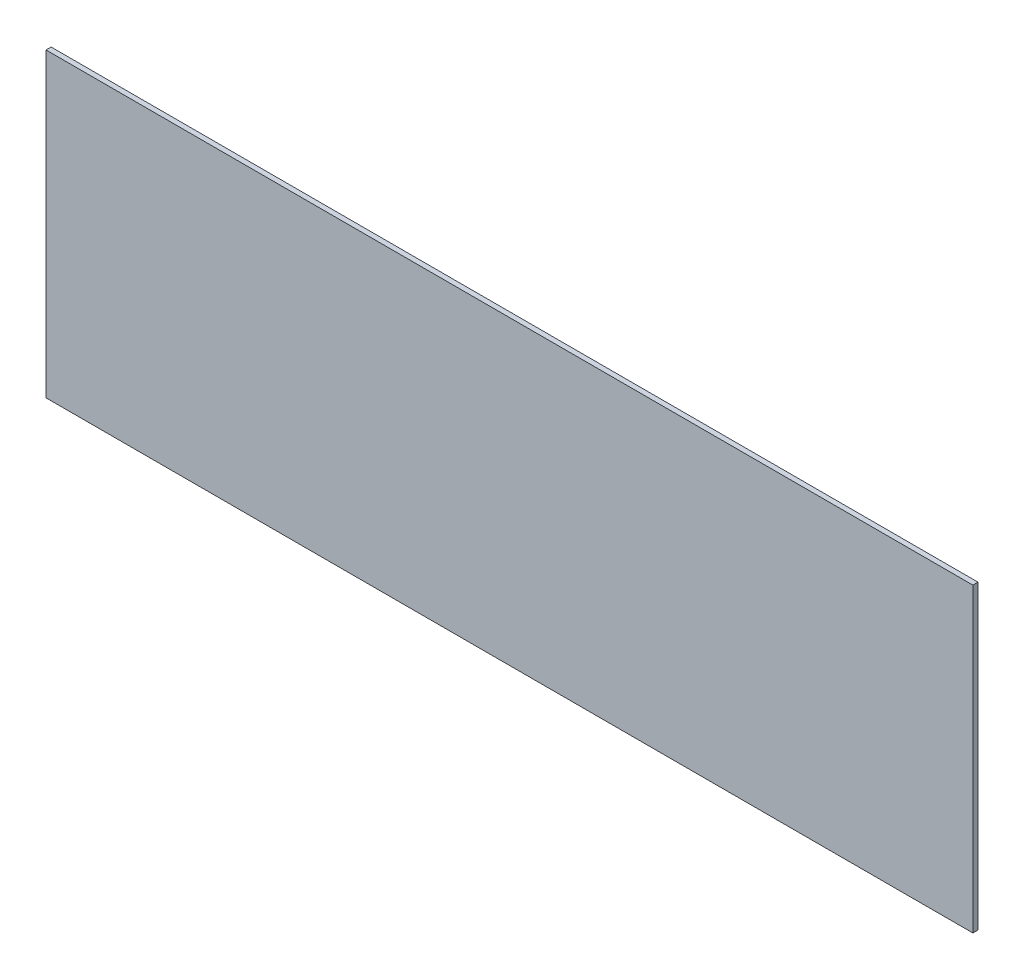
from build123d import *

# Parameters (mm, degrees)
SKETCH_1_W      = 726
SKETCH_1_H      = 236
EXTRUDE_1_DEPTH = 4


with BuildPart() as part:
    # 草图1 → 凸台-拉伸1 (new body)
    with BuildSketch(Plane.XY):
        Rectangle(SKETCH_1_W, SKETCH_1_H)
    extrude(amount=EXTRUDE_1_DEPTH)


solid = part.part
